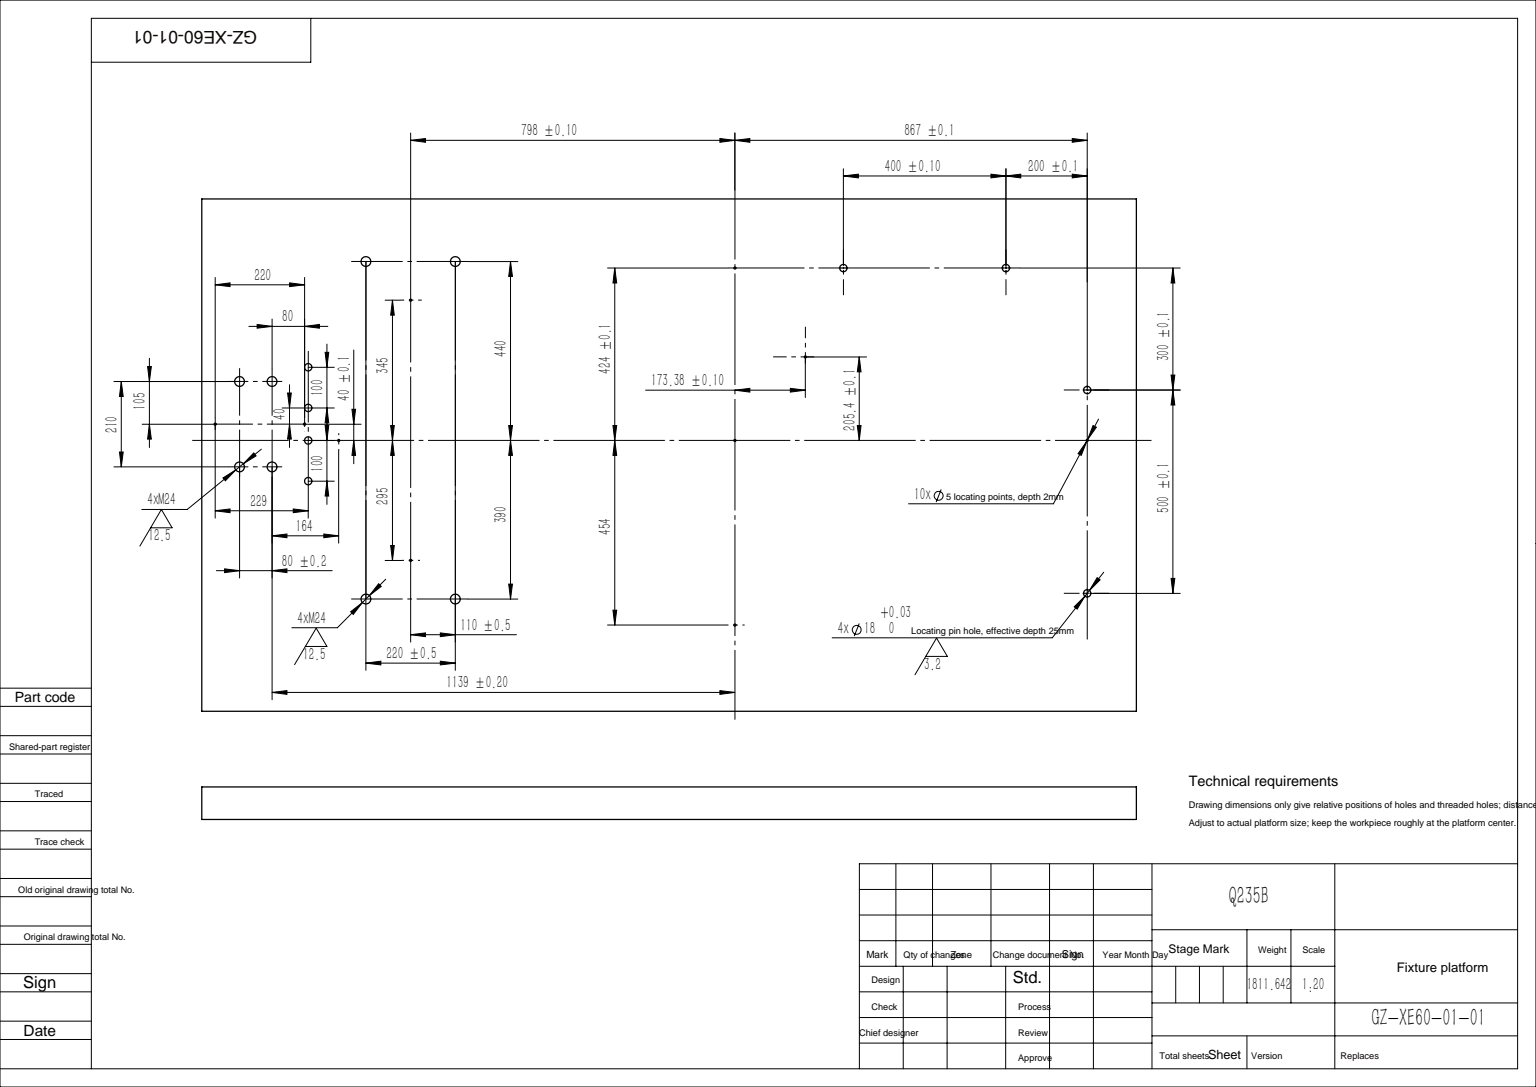
SolidWorks part; units mm, degrees
material "Q235B"
ref_plane "Front Plane" through (0, 0, 0) normal (0, 0, 1) x (1, 0, 0)
ref_plane "Top Plane" through (0, 0, 0) normal (0, 1, 0) x (1, 0, 0)
ref_plane "Right Plane" through (0, 0, 0) normal (1, 0, 0) x (0, 0, -1)
sketch "Sketch1" plane through (0, 0, 0) normal (0, 0, 1) x (1, 0, 0)
  line L0 (624, 1176.3905) -> (624, 95.9259) construction
  line L1 (0, 0) -> (2300, 0)
  line L2 (0, 0) -> (0, 1260)
  line L3 (0, 1260) -> (2300, 1260)
  line L4 (2300, 0) -> (2300, 1260)
  line L5 (-60.0931, 666) -> (2365.4814, 666) construction
  line L6 (1485.38, 1117.1638) -> (1485.38, 439.6806) construction
  line L7 (1312, 1467.2786) -> (1312, -61.2342) construction
  line L8 (1367.5318, 871.4) -> (1564.3007, 871.4) construction
  line L9 (33, 706) -> (345.5431, 706) construction
  line L10 (547.7114, 1106) -> (842.3562, 1106) construction
  line L11 (497.3237, 276) -> (825.2449, 276) construction
  line L12 (404, 1176.3905) -> (404, 231.8064) construction
  line L13 (514, 1176.3905) -> (514, 246.7682) construction
  line L14 (61.5434, 811) -> (325.7932, 811) construction
  line L15 (36.269, 601) -> (325.7932, 601) construction
  line L16 (173, 898.1187) -> (173, 506.1292) construction
  line L17 (93, 898.1187) -> (93, 506.1292) construction
  line L18 (2179, 790) -> (2179, 290) construction
  line L19 (1979, 1090) -> (1166.6774, 1090) construction
  circle A0 centre (1579, 1090) radius 9
  circle A1 centre (1979, 1090) radius 9
  circle A2 centre (2179, 790) radius 9
  circle A3 centre (2179, 290) radius 9
  circle A4 centre (93, 811) radius 12
  circle A5 centre (173, 811) radius 12
  circle A6 centre (93, 601) radius 12
  circle A7 centre (173, 601) radius 12
  circle A8 centre (404, 1106) radius 12
  circle A9 centre (624, 1106) radius 12
  circle A10 centre (404, 276) radius 12
  circle A11 centre (624, 276) radius 12
  circle A12 centre (2179, 666) radius 2.5
  circle A13 centre (337, 666) radius 2.5
  circle A14 centre (1312, 666) radius 2.5
  circle A15 centre (1485.38, 871.4) radius 2.5
  circle A16 centre (1312, 1090) radius 2.5
  circle A17 centre (1312, 212) radius 2.5
  circle A18 centre (514, 371) radius 2.5
  circle A19 centre (514, 1011) radius 2.5
  circle A20 centre (253, 706) radius 2.5
  circle A21 centre (33, 706) radius 2.5
  circle A22 centre (262, 746) radius 9
  circle A23 centre (262, 846) radius 9
  circle A24 centre (262, 666) radius 9
  circle A25 centre (262, 566) radius 9
  dimension "D3" = 170
  dimension "D4" = 18
  dimension "D5" = 18
  dimension "D6" = 121
  dimension "D7" = 200
  dimension "D8" = 400
  dimension "D9" = 300
  dimension "D10" = 500
  dimension "D11" = 424
  dimension "D12" = 693.62
  dimension "D13" = 798
  dimension "D14" = 867
  dimension "D25" = 24
  dimension "D26" = 975
  dimension "D27" = 5
  dimension "D28" = 5
  dimension "D29" = 5
  dimension "D30" = 5
  dimension "D31" = 5
  dimension "D32" = 454
  dimension "D33" = 5
  dimension "D34" = 95
  dimension "D35" = 5
  dimension "D36" = 5
  dimension "D37" = 95
  dimension "D38" = 5
  dimension "D39" = 5
  dimension "D40" = 60
  dimension "D42" = 18
  dimension "D43" = 89
  dimension "D44" = 100
  dimension "D45" = 100
  dimension "D46" = 40
  dimension "D47" = 40
  dimension "D1" = 2300
  dimension "D2" = 1260
  dimension "D15" = 205.4
  dimension "D16" = 40
  dimension "D17" = 390
  dimension "D18" = 440
  dimension "D19" = 110
  dimension "D20" = 220
  dimension "D21" = 210
  dimension "D22" = 105
  dimension "D23" = 1139
  dimension "D24" = 80
  dimension "D41" = 80
extrude "Boss-Extrude1" add sketch "Sketch1" along normal blind 80
